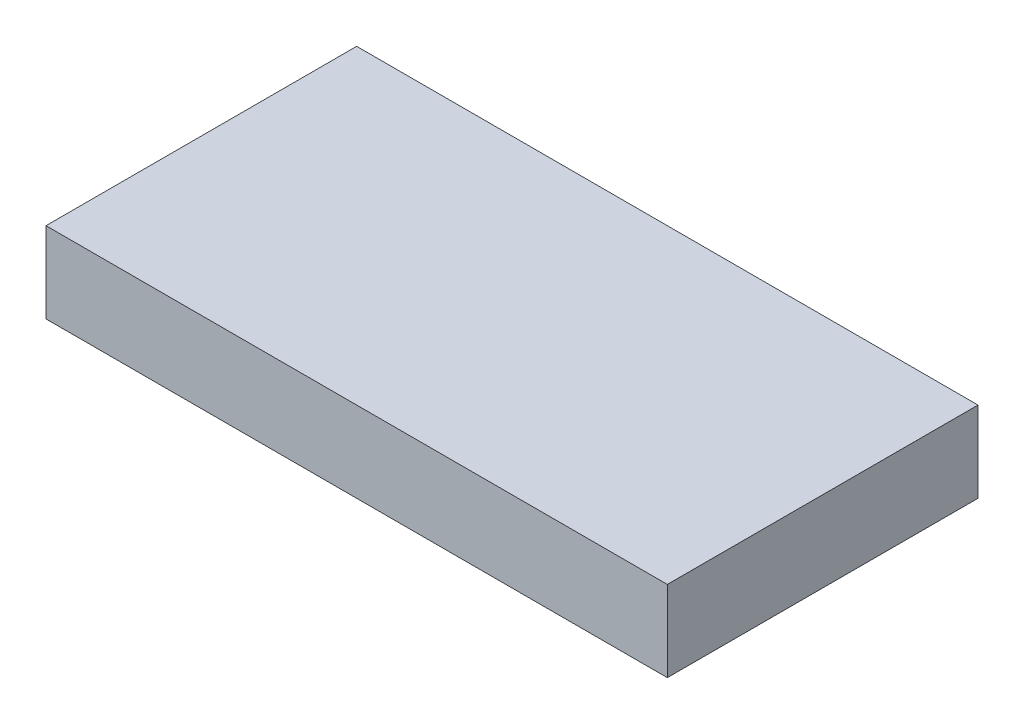
from build123d import *

# Parameters (mm, degrees)
SKETCH1_W           = 20
SKETCH1_H           = 10
BOSS_EXTRUDE1_DEPTH = 2.6


with BuildPart() as part:
    # Sketch1 → Boss-Extrude1 (new body)
    with BuildSketch(Plane(origin=(0, 0, 0), x_dir=(1, 0, 0), z_dir=(0, 1, 0))):
        Rectangle(SKETCH1_W, SKETCH1_H)
    extrude(amount=BOSS_EXTRUDE1_DEPTH)


solid = part.part
